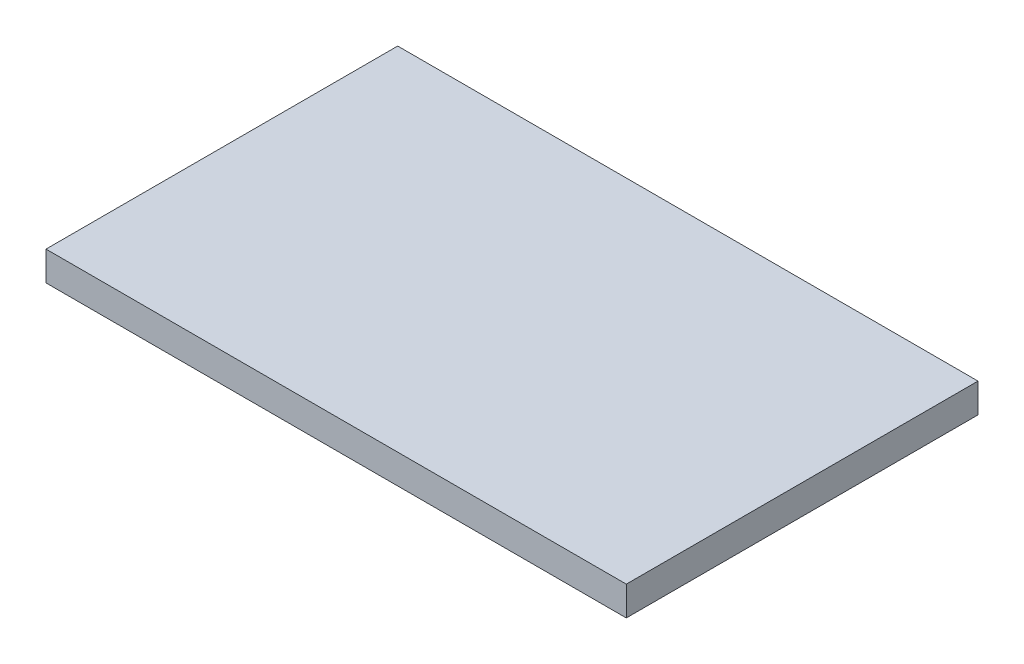
SolidWorks part; units mm, degrees
ref_plane "前视基准面" through (0, 0, 0) normal (0, 0, 1) x (1, 0, 0)
ref_plane "上视基准面" through (0, 0, 0) normal (0, 1, 0) x (1, 0, 0)
ref_plane "右视基准面" through (0, 0, 0) normal (1, 0, 0) x (0, 0, -1)
sketch "草图1" plane through (0, 0, 0) normal (0, 0, 1) x (1, 0, 0)
  line L1 (-49.5, -2.5) -> (49.5, -2.5)
  line L2 (-49.5, -2.5) -> (-49.5, 2.5)
  line L3 (-49.5, 2.5) -> (49.5, 2.5)
  line L4 (49.5, -2.5) -> (49.5, 2.5)
  line L5 (-49.5, -2.5) -> (49.5, 2.5) construction
  line L6 (-49.5, 2.5) -> (49.5, -2.5) construction
  point P0 (0, 0)
  dimension "D1" = 99
  dimension "D2" = 5
extrude "凸台-拉伸1" add sketch "草图1" along normal mid plane 60
